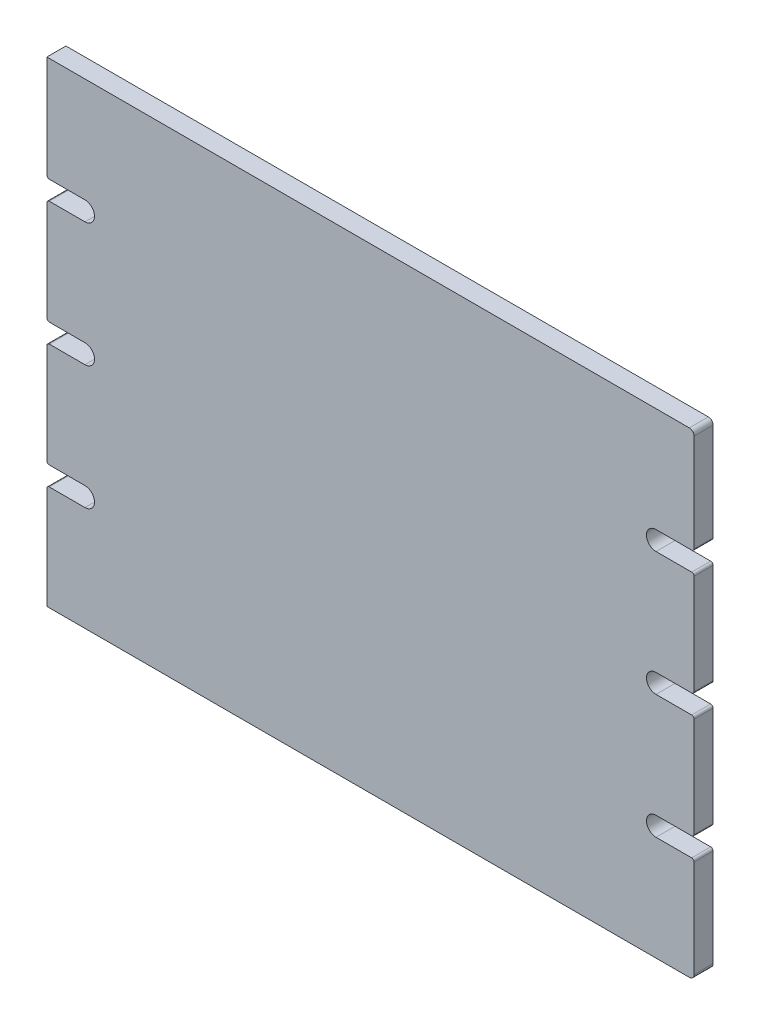
SolidWorks part; units mm, degrees
material "Q235B"
ref_plane "Front Plane" through (0, 0, 0) normal (0, 0, 1) x (1, 0, 0)
ref_plane "Top Plane" through (0, 0, 0) normal (0, 1, 0) x (1, 0, 0)
ref_plane "Right Plane" through (0, 0, 0) normal (1, 0, 0) x (0, 0, -1)
sketch "Sketch1" plane through (0, 0, 0) normal (0, 0, 1) x (1, 0, 0)
  line L0 (0, 780) -> (80, 780)
  line L1 (0, 0) -> (1360, 0)
  line L2 (0, 0) -> (0, 220)
  line L3 (0, 1000) -> (1360, 1000)
  line L4 (1360, 0) -> (1360, 220)
  line L5 (80, 740) -> (0, 740)
  line L6 (1360, 780) -> (1280, 780)
  line L7 (1280, 740) -> (1360, 740)
  line L8 (80, 480) -> (0, 480)
  line L9 (0, 520) -> (80, 520)
  line L10 (1280, 480) -> (1360, 480)
  line L11 (1360, 520) -> (1280, 520)
  line L12 (80, 220) -> (0, 220)
  line L13 (0, 260) -> (80, 260)
  line L14 (1280, 220) -> (1360, 220)
  line L15 (1360, 260) -> (1280, 260)
  line L16 (0, 780) -> (0, 1000)
  line L17 (0, 520) -> (0, 740)
  line L18 (0, 260) -> (0, 480)
  line L19 (1360, 260) -> (1360, 480)
  line L20 (1360, 520) -> (1360, 740)
  line L21 (1360, 780) -> (1360, 1000)
  arc A0 (80, 780) -> (80, 740) centre (80, 760) cw
  arc A1 (1280, 780) -> (1280, 740) centre (1280, 760) ccw
  arc A2 (80, 520) -> (80, 480) centre (80, 500) cw
  arc A3 (1280, 520) -> (1280, 480) centre (1280, 500) ccw
  arc A4 (80, 260) -> (80, 220) centre (80, 240) cw
  arc A5 (1280, 260) -> (1280, 220) centre (1280, 240) ccw
  dimension "D1" = 1360
  dimension "D2" = 1000
  dimension "D3" = 40
  dimension "D4" = 220
  dimension "D5" = 80
  dimension "D6" = 40
  dimension "D7" = 80
  dimension "D8" = 3
extrude "Boss-Extrude1" add sketch "Sketch1" along normal blind 40
fillet "Fillet1" radius 5 12 edges at (1360, 780, 20) (1360, 740, 20) (1360, 480, 20) (1360, 520, 20) (1360, 260, 20) (1360, 220, 20) (0, 220, 20) (0, 260, 20) (0, 480, 20) (0, 520, 20) (0, 740, 20) (0, 780, 20)
fillet "Fillet2" radius 10 2 edges at (1360, 1000, 20) (1360, 0, 20)
